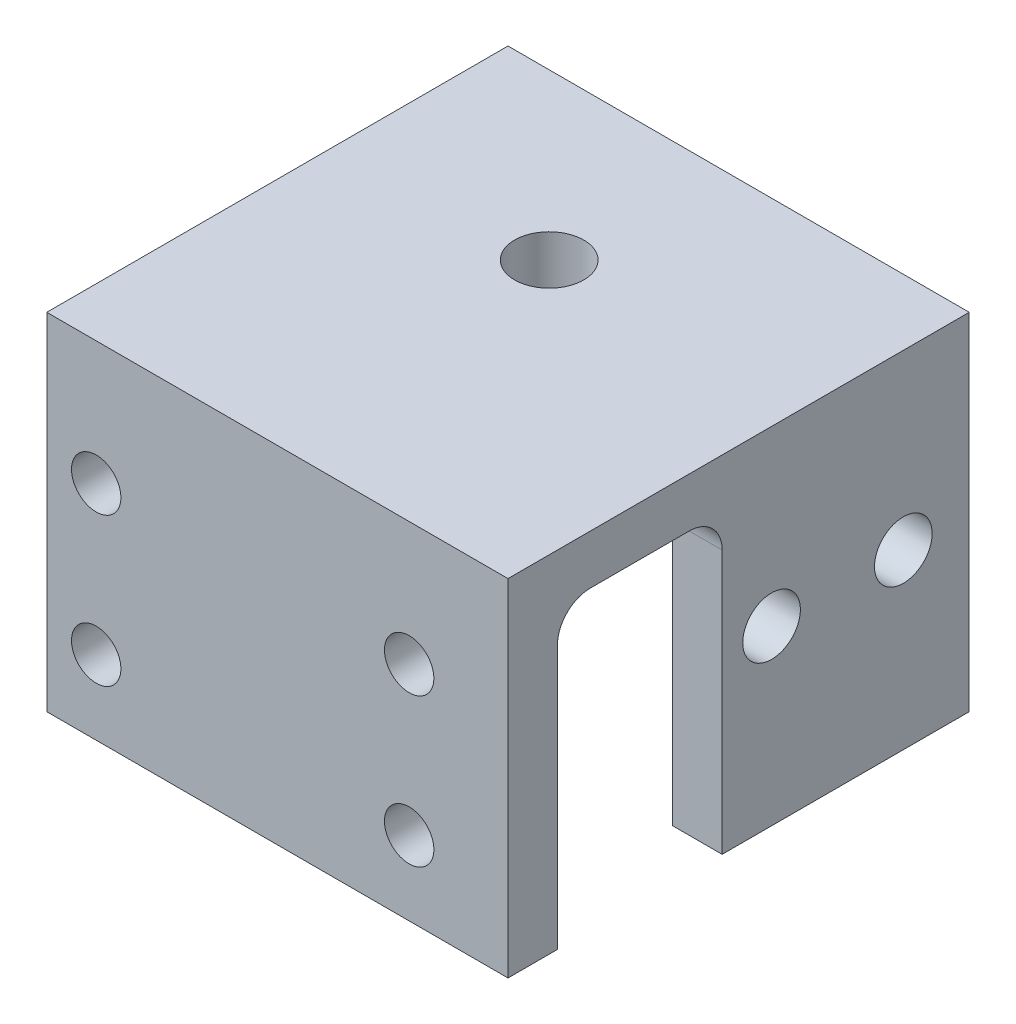
SolidWorks part; units mm, degrees
ref_plane "Front Plane" through (0, 0, 0) normal (0, 0, 1) x (1, 0, 0)
ref_plane "Top Plane" through (0, 0, 0) normal (0, 1, 0) x (1, 0, 0)
ref_plane "Right Plane" through (0, 0, 0) normal (1, 0, 0) x (0, 0, -1)
sketch "Sketch1" plane through (0, 0, 0) normal (0, 0, 1) x (1, 0, 0)
  line L1 (-12.5, -9) -> (12.5, -9)
  line L2 (-12.5, -9) -> (-12.5, 9)
  line L3 (-12.5, 9) -> (12.5, 9)
  line L4 (12.5, -9) -> (12.5, 9)
  line L5 (-12.5, -9) -> (12.5, 9) construction
  line L6 (-12.5, 9) -> (12.5, -9) construction
  circle A0 centre (-9.5, 4.5) radius 1.5
  circle A1 centre (9.5, 4.5) radius 1.5
  circle A2 centre (9.5, -4.5) radius 1.5
  circle A3 centre (-9.5, -4.5) radius 1.5
  point P0 (0, 0)
  dimension "D2" = 3
  dimension "D3" = 3
  dimension "D8" = 3
  dimension "D9" = 3
  dimension "D10" = 19
  dimension "D13" = 3
  dimension "D1" = 18
  dimension "D4" = 4.5
  dimension "D5" = 4.5
  dimension "D6" = 4.5
  dimension "D7" = 9
  dimension "D11" = 25
  dimension "D12" = 3
  dimension "D14" = 19
extrude "Boss-Extrude1" add sketch "Sketch1" along normal blind 3
sketch "Sketch2" plane through (0, 9, 0) normal (0, 1, 0) x (1, 0, 0)
  line L0 (12.5, 0) -> (-12.5, 0) construction
  line L1 (-12.5, -3) -> (12.5, -3)
  line L2 (-12.5, -3) -> (-12.5, 25)
  line L3 (-12.5, 25) -> (12.5, 25)
  line L4 (12.5, -3) -> (12.5, 25)
  circle A0 centre (0, 15) radius 2.1
  dimension "D2" = 4.2
  dimension "D1" = 25
  dimension "D3" = 10
extrude "Boss-Extrude2" add sketch "Sketch2" along normal blind 3
sketch "Sketch3" plane through (12.5, 0, 0) normal (-1, 0, 0) x (0, 0, 1)
  line L0 (0, -9) -> (0, 7)
  line L1 (3, 12) -> (-25, 12)
  line L2 (3, 12) -> (3, -9)
  line L3 (3, -9) -> (0, -9)
  line L4 (-25, 12) -> (-25, -9)
  line L5 (-10, 7) -> (-10, -9)
  line L6 (0, 9) -> (-25, 9) construction
  line L7 (-10, -9) -> (-25, -9)
  line L8 (-8, 9) -> (-2, 9)
  arc A0 (-2, 9) -> (0, 7) centre (-2, 7) cw
  arc A1 (-8, 9) -> (-10, 7) centre (-8, 7) ccw
  circle A2 centre (-21, 1.5) radius 1.75
  circle A3 centre (-13, 1.5) radius 1.75
  point P15 (0, 9)
  point P18 (-10, 9)
  dimension "D4" = 2
  dimension "D5" = 3.5
  dimension "D6" = 3.5
  dimension "D8" = 10.5
  dimension "D10" = 3
  dimension "D9" = 8
  dimension "D1" = 21
  dimension "D2" = 28
  dimension "D3" = 10
  dimension "D7" = 7.5
extrude "Boss-Extrude3" add sketch "Sketch3" against normal blind 3
